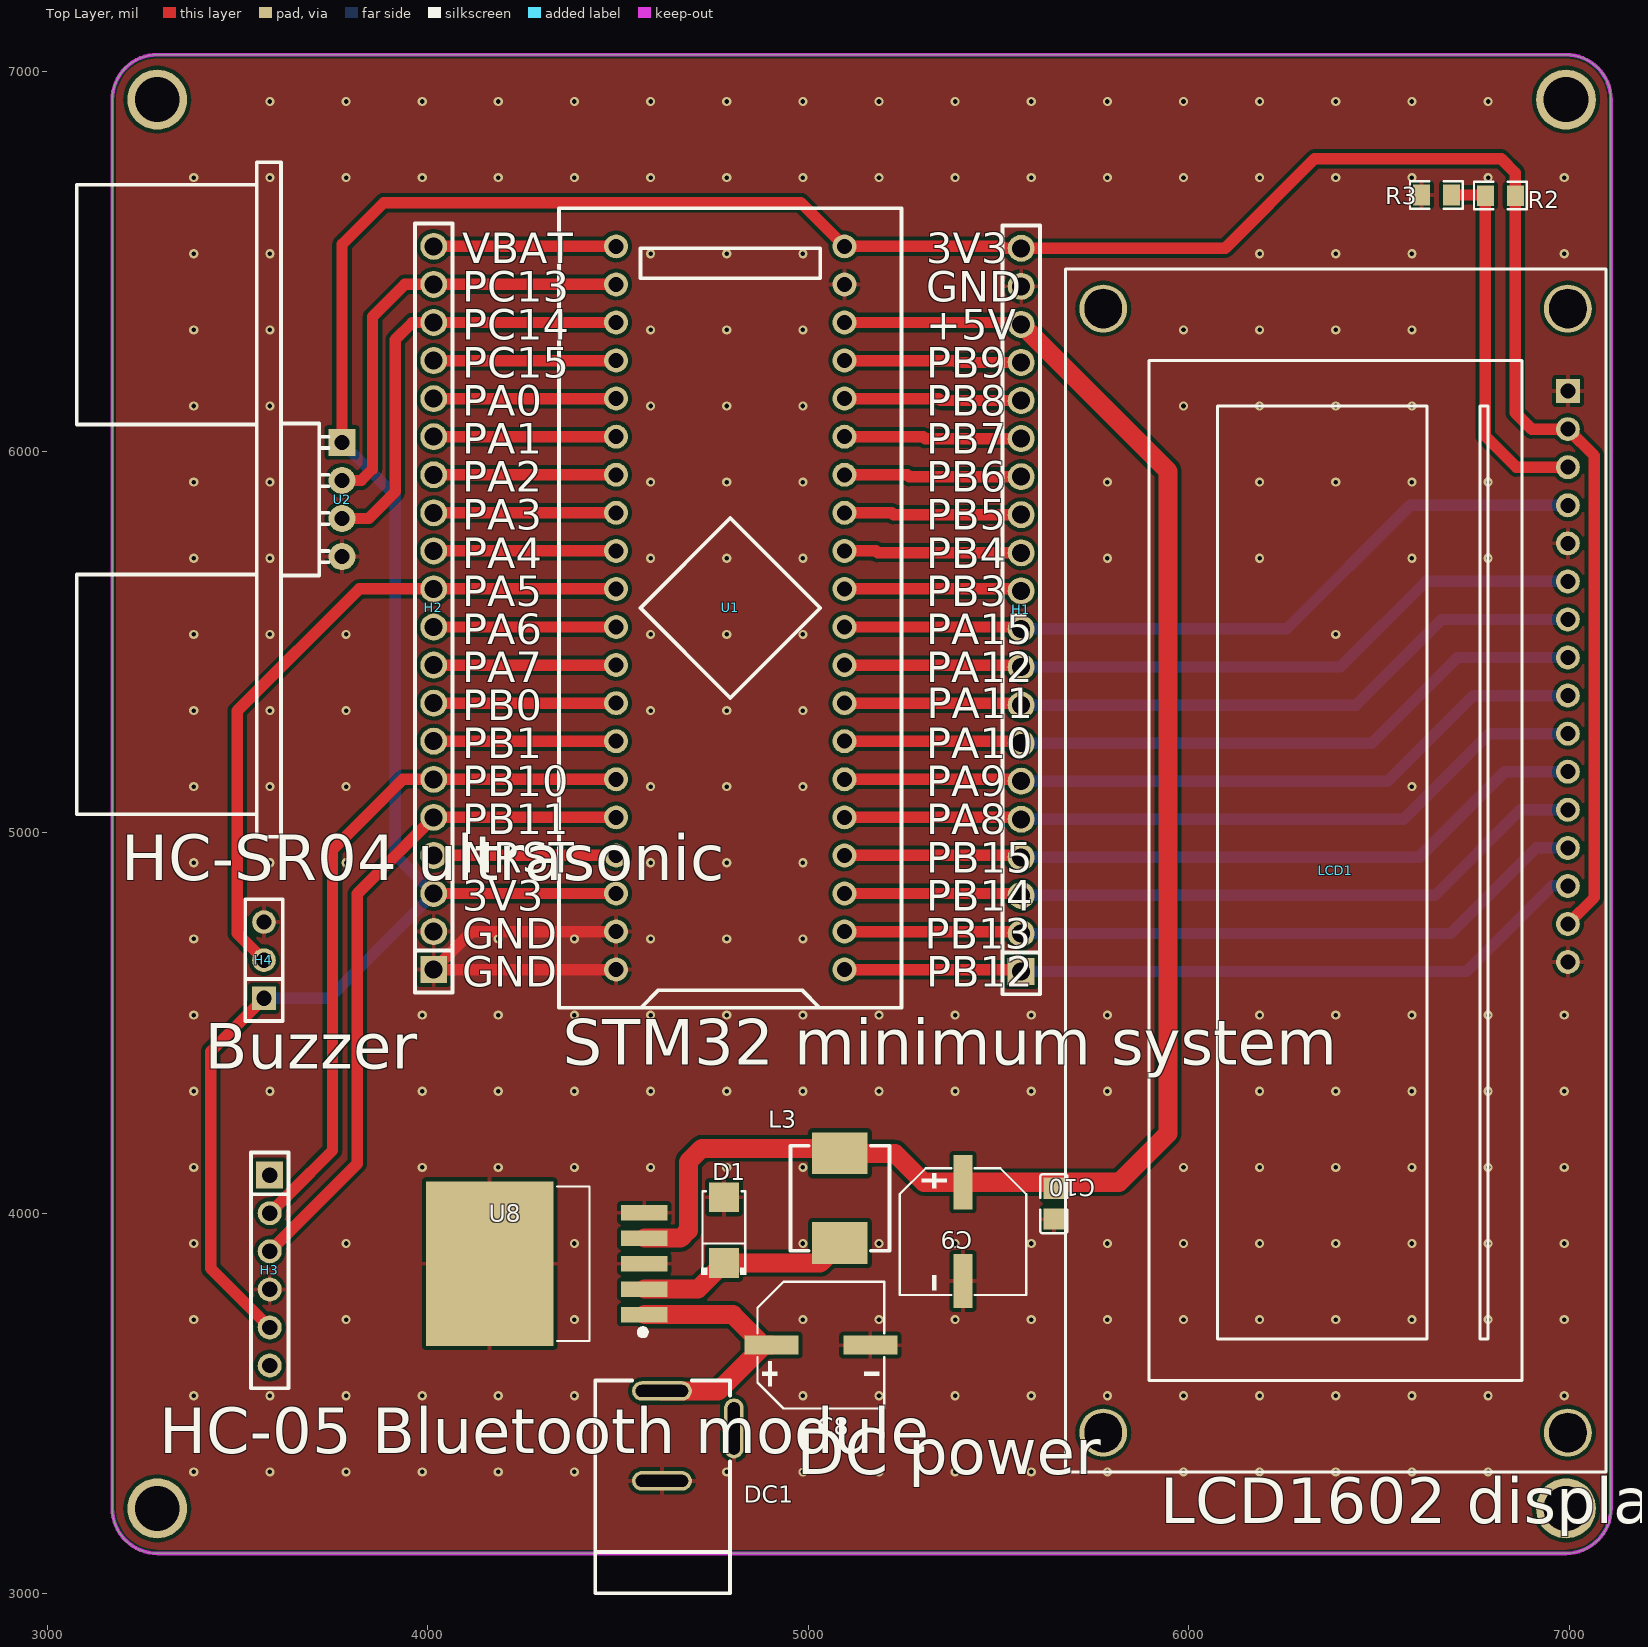
[diagram p0: Top Layer view]
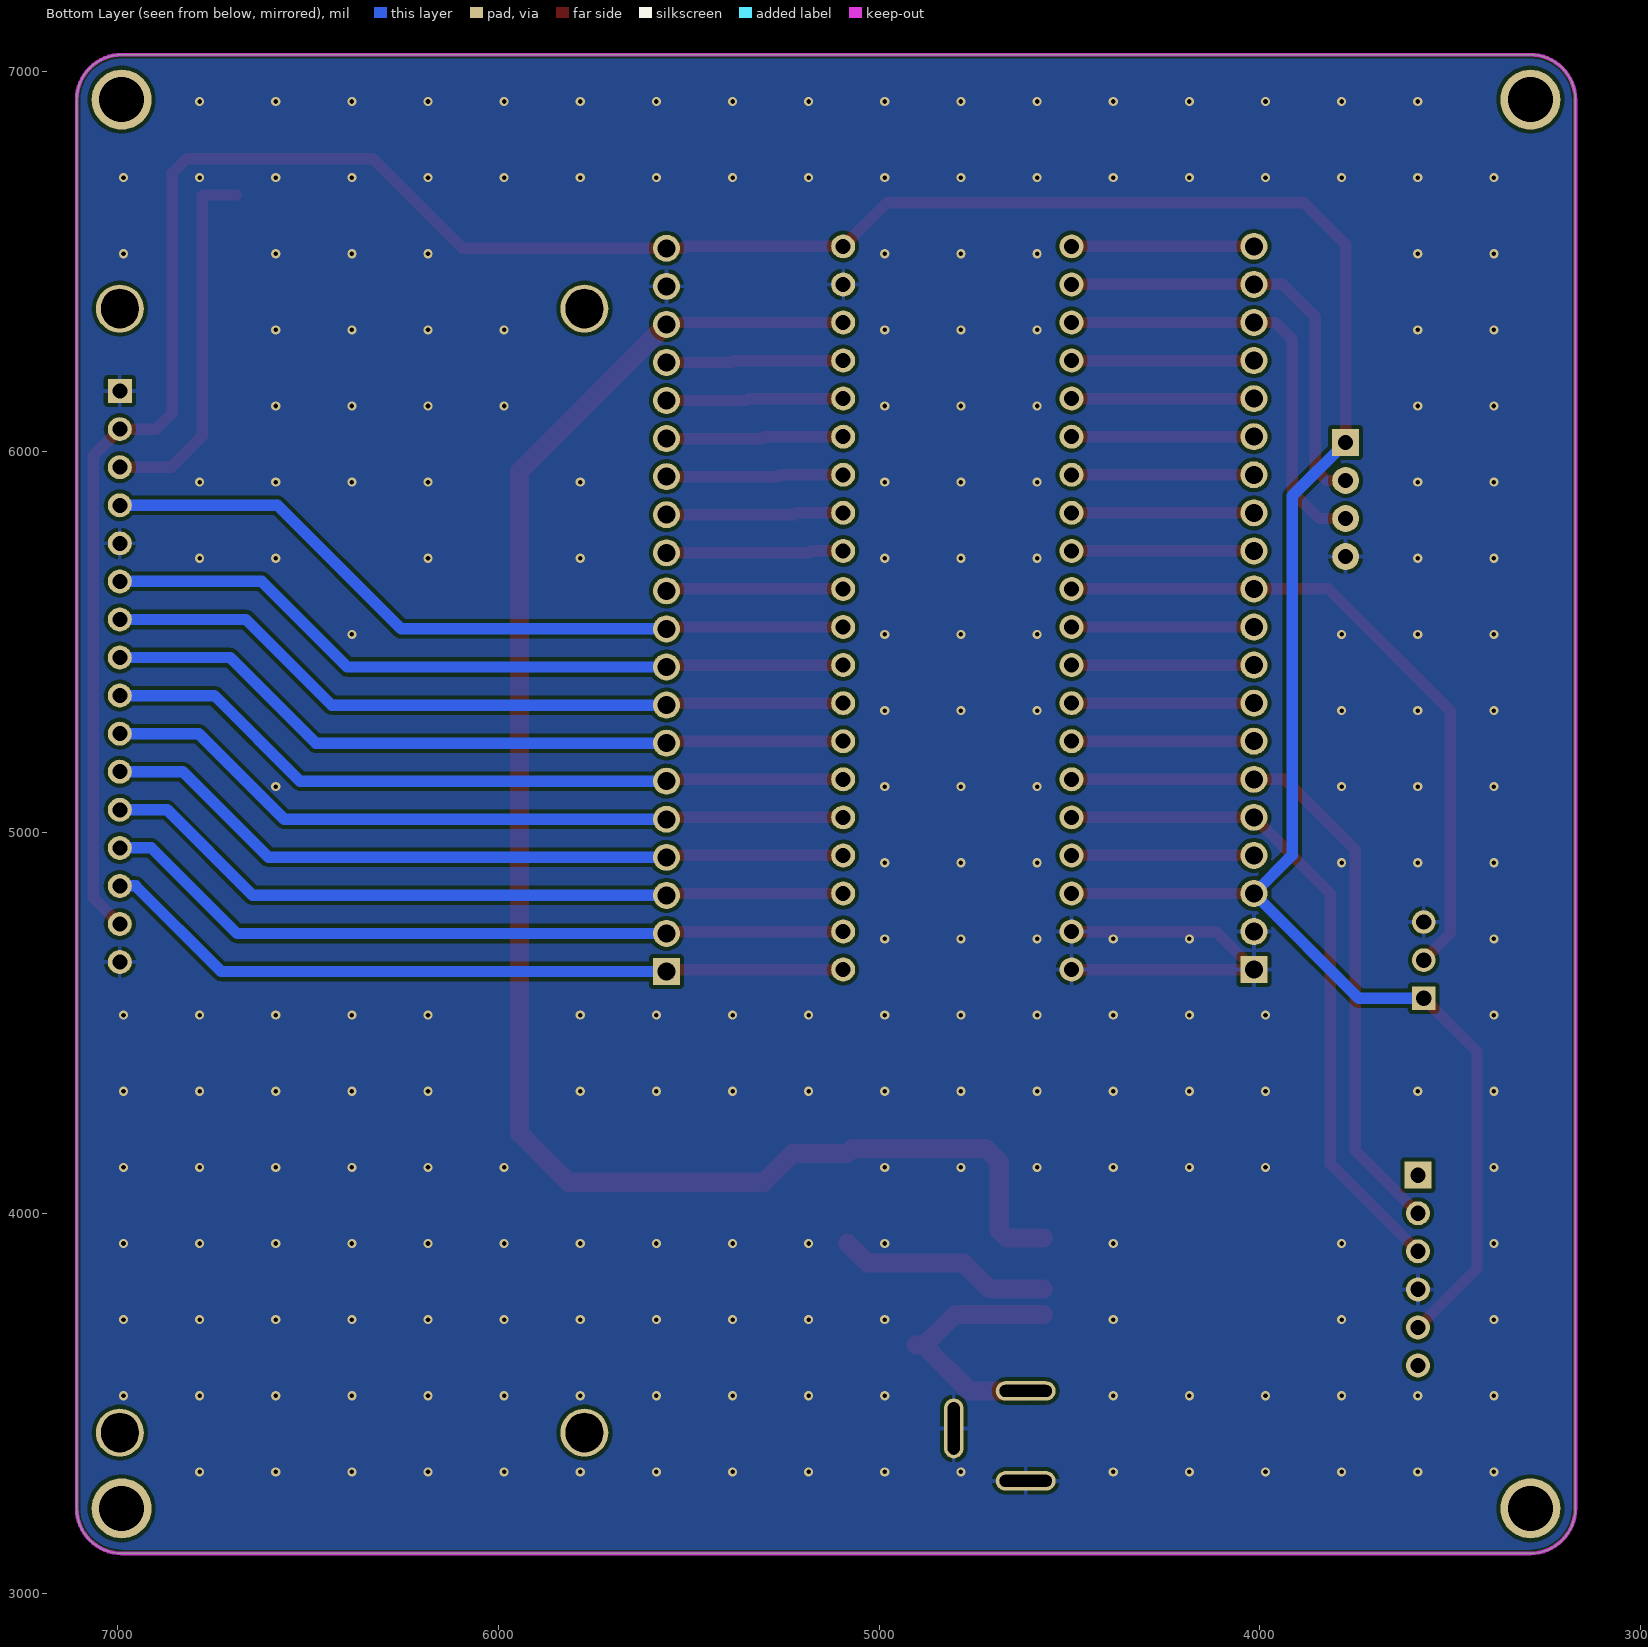
[diagram p1: Bottom Layer view, seen from below]
# Altium PCB MISC89129.pcbdoc
Units mil, origin at the board's own origin, x right, y up, seen from the top; angles counter-clockwise.
Board outline 3937.01 x 3937.01 mil, 2 copper layers (Top Layer, Bottom Layer), stack 62.206 mil thick; 16 components, 40 nets, 140 pads, 222 vias.

## Layer stack, top to bottom
Top Solder Mask Layer: solder mask 0.394, Dk 3.3
Top Layer: signal copper 1.379
Dielectric1: surface 59.449, FR4, Dk 4.5
Bottom Layer: signal copper 1.378
Bottom Solder Mask Layer: solder mask 0.394, Dk 3.3

## Board outline
3289.61,7043.5 ccw(c3289.61,6925.39) 3171.5,6925.39 3171.5,3224.61 ccw(c3289.61,3224.61) 3289.61,3106.5 6990.39,3106.5 ccw(c6990.39,3224.61) 7108.5,3224.61 7108.5,6925.39 ccw(c6990.39,6925.39) 6990.39,7043.5 3289.61,7043.5

## Design rules (kind name [scope] priority, off if disabled: settings)
BoardOutlineClearance copperThickness2oz_1 [All] p2 off: genericclearance=7.99 ignorepadtopadclearanceinfootprint=FALSE except(0: Arc-SplitContinuation Track-SplitContinuation SMDPad-SplitContinuation THPad-SplitContinuation Via-SplitContinuation Fill-SplitContinuation Region-SplitContinuation Poly-SplitContinuation Text-SplitContinuation Hole-SplitContinuation; 5.98: Arc-CutoutEdge Track-CutoutEdge SMDPad-CutoutEdge THPad-CutoutEdge Via-CutoutEdge Text-CutoutEdge; 6.9: Hole-OutlineEdge Hole-CutoutEdge; 10: Poly-OutlineEdge Poly-CutoutEdge; 11.81: Arc-OutlineEdge Track-OutlineEdge SMDPad-OutlineEdge THPad-OutlineEdge Via-OutlineEdge Fill-OutlineEdge Region-OutlineEdge Text-OutlineEdge Fill-CutoutEdge Region-CutoutEdge)
BoardOutlineClearance Plane_innerPlane_1 [All] p4 off: genericclearance=4.02 ignorepadtopadclearanceinfootprint=FALSE except(0: Arc-SplitContinuation Track-SplitContinuation SMDPad-SplitContinuation THPad-SplitContinuation Via-SplitContinuation Fill-SplitContinuation Region-SplitContinuation Poly-SplitContinuation Text-SplitContinuation Hole-SplitContinuation; 5.98: Arc-CutoutEdge Track-CutoutEdge SMDPad-CutoutEdge THPad-CutoutEdge Via-CutoutEdge Text-CutoutEdge; 6.9: Hole-OutlineEdge Hole-CutoutEdge; 10: Poly-OutlineEdge Poly-CutoutEdge; 11.81: Arc-OutlineEdge Track-OutlineEdge SMDPad-OutlineEdge THPad-OutlineEdge Via-OutlineEdge Fill-OutlineEdge Region-OutlineEdge Text-OutlineEdge Fill-CutoutEdge Region-CutoutEdge)
BoardOutlineClearance Copper_copperRegion_1 [All] p6 off: genericclearance=4.02 ignorepadtopadclearanceinfootprint=FALSE except(0: Arc-SplitContinuation Track-SplitContinuation SMDPad-SplitContinuation THPad-SplitContinuation Via-SplitContinuation Fill-SplitContinuation Region-SplitContinuation Poly-SplitContinuation Text-SplitContinuation Hole-SplitContinuation; 5.98: Arc-CutoutEdge Track-CutoutEdge SMDPad-CutoutEdge THPad-CutoutEdge Via-CutoutEdge Text-CutoutEdge; 6.9: Hole-OutlineEdge Hole-CutoutEdge; 10: Poly-OutlineEdge Poly-CutoutEdge; 11.81: Arc-OutlineEdge Track-OutlineEdge SMDPad-OutlineEdge THPad-OutlineEdge Via-OutlineEdge Fill-OutlineEdge Region-OutlineEdge Text-OutlineEdge Fill-CutoutEdge Region-CutoutEdge)
BoardOutlineClearance copperThickness1oz_1 [All] p8: genericclearance=4.02 ignorepadtopadclearanceinfootprint=FALSE except(0: Arc-SplitContinuation Track-SplitContinuation SMDPad-SplitContinuation THPad-SplitContinuation Via-SplitContinuation Fill-SplitContinuation Region-SplitContinuation Poly-SplitContinuation Text-SplitContinuation Hole-SplitContinuation; 5.98: Arc-CutoutEdge Track-CutoutEdge SMDPad-CutoutEdge THPad-CutoutEdge Via-CutoutEdge Text-CutoutEdge; 6.9: Hole-OutlineEdge Hole-CutoutEdge; 10: Poly-OutlineEdge Poly-CutoutEdge; 11.81: Arc-OutlineEdge Track-OutlineEdge SMDPad-OutlineEdge THPad-OutlineEdge Via-OutlineEdge Fill-OutlineEdge Region-OutlineEdge Text-OutlineEdge Fill-CutoutEdge Region-CutoutEdge)
Clearance copperThickness2oz [All] p1 off: gap=7.99 ignorepadtopadclearanceinfootprint=FALSE except(5.98: SMDPad-Track SMDPad-SMDPad THPad-Track SMDPad-THPad THPad-THPad Track-Via SMDPad-Via THPad-Via Via-Via Fill-SMDPad Region-SMDPad Fill-THPad Region-THPad Fill-Via Region-Via Fill-Fill Fill-Region Region-Region Arc-Track Arc-SMDPad Arc-THPad Arc-Via Fill-Arc Region-Arc Arc-Arc Text-Track SMDPad-Text Text-THPad Text-Via Fill-Text Region-Text Arc-Text Text-Text; 6.9: Hole-Track Hole-SMDPad Hole-THPad Hole-Via Fill-Hole Region-Hole Hole-Arc Hole-Text; 10: Poly-Track Poly-SMDPad Poly-THPad Poly-Via Poly-Fill Poly-Region Poly-Poly Poly-Arc Poly-Text Poly-Hole; 11.81: Fill-Track Region-Track)
Clearance Plane_innerPlane [All] p3 off: gap=4.02 ignorepadtopadclearanceinfootprint=FALSE except(5.98: SMDPad-Track SMDPad-SMDPad THPad-Track SMDPad-THPad THPad-THPad Track-Via SMDPad-Via THPad-Via Via-Via Fill-SMDPad Region-SMDPad Fill-THPad Region-THPad Fill-Via Region-Via Fill-Fill Fill-Region Region-Region Arc-Track Arc-SMDPad Arc-THPad Arc-Via Fill-Arc Region-Arc Arc-Arc Text-Track SMDPad-Text Text-THPad Text-Via Fill-Text Region-Text Arc-Text Text-Text; 6.9: Hole-Track Hole-SMDPad Hole-THPad Hole-Via Fill-Hole Region-Hole Hole-Arc Hole-Text; 10: Poly-Track Poly-SMDPad Poly-THPad Poly-Via Poly-Fill Poly-Region Poly-Poly Poly-Arc Poly-Text Poly-Hole; 11.81: Fill-Track Region-Track)
Clearance Copper_copperRegion [All] p5 off: gap=4.02 ignorepadtopadclearanceinfootprint=FALSE except(5.98: SMDPad-Track SMDPad-SMDPad THPad-Track SMDPad-THPad THPad-THPad Track-Via SMDPad-Via THPad-Via Via-Via Fill-SMDPad Region-SMDPad Fill-THPad Region-THPad Fill-Via Region-Via Fill-Fill Fill-Region Region-Region Arc-Track Arc-SMDPad Arc-THPad Arc-Via Fill-Arc Region-Arc Arc-Arc Text-Track SMDPad-Text Text-THPad Text-Via Fill-Text Region-Text Arc-Text Text-Text; 6.9: Hole-Track Hole-SMDPad Hole-THPad Hole-Via Fill-Hole Region-Hole Hole-Arc Hole-Text; 10: Poly-Track Poly-SMDPad Poly-THPad Poly-Via Poly-Fill Poly-Region Poly-Poly Poly-Arc Poly-Text Poly-Hole; 11.81: Fill-Track Region-Track)
Clearance copperThickness1oz [All] p7: gap=4.02 ignorepadtopadclearanceinfootprint=FALSE except(5.98: SMDPad-Track SMDPad-SMDPad THPad-Track SMDPad-THPad THPad-THPad Track-Via SMDPad-Via THPad-Via Via-Via Fill-SMDPad Region-SMDPad Fill-THPad Region-THPad Fill-Via Region-Via Fill-Fill Fill-Region Region-Region Arc-Track Arc-SMDPad Arc-THPad Arc-Via Fill-Arc Region-Arc Arc-Arc Text-Track SMDPad-Text Text-THPad Text-Via Fill-Text Region-Text Arc-Text Text-Text; 6.9: Hole-Track Hole-SMDPad Hole-THPad Hole-Via Fill-Hole Region-Hole Hole-Arc Hole-Text; 10: Poly-Track Poly-SMDPad Poly-THPad Poly-Via Poly-Fill Poly-Region Poly-Poly Poly-Arc Poly-Text Poly-Hole; 11.81: Fill-Track Region-Track)
DiffPairsRouting differentialPair [All] p1: maxlimit=6 minlimit=6 mostfreqgap=6 toplayer_minwidth=5 toplayer_prefwidth=10 toplayer_maxwidth=100 toplayer_mingap=6 toplayer_prefgap=6 toplayer_maxgap=6 bottomlayer_minwidth=5 bottomlayer_prefwidth=10 bottomlayer_maxwidth=100 bottomlayer_mingap=6 bottomlayer_prefgap=6 bottomlayer_maxgap=6 maxuncoupledlength=10
HoleToHoleClearance otherClearance [All] p1: gap=11.81 allowstackedmicrovias=TRUE
Length netLength [All] p1: minlimit=0 maxlimit=0
PasteMaskExpansion pasteMaskExpansion [All] p1: expansion=0
PlaneConnect innerPlane [All] p1: planeconnectstyle=Relief reliefexpansion=20 reliefentries=4 reliefconductorwidth=10 reliefairgap=10
PolygonConnect copperRegion [All] p1: connectstyle=Relief reliefconductorwidth=10 reliefentries=4 polygonreliefangle="90 Angle" airgapwidth=10 via.connectstyle=Relief via.reliefconductorwidth=10 via.reliefentries=4 via.polygonreliefangle="90 Angle" via.airgapwidth=10
RoutingVias viaSize [All] p1: holewidth=12.01 width=24.02 viastyle="Through Hole" minholewidth=11.81 minwidth=19.68 maxholewidth=248.03 maxwidth=393.7
SolderMaskExpansion solderMaskExpansion [IsVia] p1: expansion=-1000 istentingtop=TRUE
SolderMaskExpansion solderMaskExpansion [All] p2: expansion=2 istentingtop=FALSE
Width copperThickness2oz_2 [All] p1 off: maxlimit=100 minlimit=8 preferedwidth=10
Width copperThickness1oz_2 [All] p2: maxlimit=100 minlimit=5 preferedwidth=10

## Components (designator, comment, footprint, x,y, rotation, side; value= is the part's Value field where it differs from the comment)
C8 "" CAP-SMD_BD8.0-L8.3-W8.3-RD 5033.1,3653.46 r180 top
C9 "" CAP-SMD_BD8.0-L8.3-W8.3-RD 5406.18,3951.73 r90 top
C10 "" C0805 5645,4025 r270 top
D1 "" SMA_L4.3-W2.6-LS5.2-RD 4778.1,3955.46 r90 top
DC1 "" DC-2.0 4605,3410 r270 top
H1 "" HDR-TH_20P-P2.54-V-F 5559.16,5585 r90 top
H2 "" HDR-TH_20P-P2.54-V-F 4015.95,5590 r90 top
H3 "" HDR-TH_6P-P2.54-V-F 3585,3850 r270 top
H4 "" HDR-TH_3P-P2.54-V-F 3570,4665 r90 top
L3 "" IND-SMD_L7.0-W6.6 5083.1,4039.46 r90 top
LCD1 "LMB162ADC" LCD1602 6385,4900 r270 top
R2 "10K" R0805 6817.76,6673.32 r0 top
R3 "1K" R0805 6650,6675 r0 top
U1 "STM32F103C8T6-Card" CONN-TH_L53.3-W22.9_STM32F103C8T6-CARD 4795,5590 r90 top
U2 "HC-SR04" TH_HC-SR04V 3775,5875 r270 top
U8 "LM2596S-5.0" TO-263-5_L10.2-W8.9-P1.70-BR 4365.96,3867.46 r0 top

## Footprints (in the part's own frame and the unit in brackets; to place one, negate y for a bottom-side part, rotate by r counter-clockwise, add the part's x,y. Pads: shape width x height; smd on the part's side, far side on the other; paste and mask are expansions set on the pad)
C0805 [mm]
  rect 1.41x1.35 smd paste-100 mask+0.051: 1(-1.03,0) 2(1.03,0)
  silkscreen extent -1.96,-0.9 1.96,0.9
CAP-SMD_BD8.0-L8.3-W8.3-RD [mm]
  rect 3.61x1.26 smd paste+0 mask+0.051: 1(3.295,0) 2(-3.295,0)
  silkscreen extent -4.23,-4.23 4.23,4.23
CONN-TH_L53.3-W22.9_STM32F103C8T6-CARD [mm]
  round 1.6 hole 1: 1(-24.13,-7.62) 2(-21.59,-7.62) 3(-19.05,-7.62) 4(-16.51,-7.62) 5(-13.97,-7.62) 6(-11.43,-7.62) 7(-8.89,-7.62) 8(-6.35,-7.62) 9(-3.81,-7.62) 10(-1.27,-7.62) 11(1.27,-7.62) 12(3.81,-7.62) 13(6.35,-7.62) 14(8.89,-7.62) 15(11.43,-7.62) 16(13.97,-7.62) 17(16.51,-7.62) 18(19.05,-7.62) 19(21.59,-7.62) 20(24.13,-7.62) 21(24.13,7.62) 22(21.59,7.62) 23(19.05,7.62) 24(16.51,7.62) 25(13.97,7.62) 26(11.43,7.62) 27(8.89,7.62) 28(6.35,7.62) 29(3.81,7.62) 30(1.27,7.62) 31(-1.27,7.62) 32(-3.81,7.62) 33(-6.35,7.62) 34(-8.89,7.62) 35(-11.43,7.62) 36(-13.97,7.62) 37(-16.51,7.62) 38(-19.05,7.62) 39(-21.59,7.62) 40(-24.13,7.62)
  silkscreen extent -26.67,-11.43 26.67,11.43
DC-2.0 [mil]
  oval 157.5x51.2 hole 31.5 slot 137.8 at 0 deg paste+0 mask+2: 2(-24.7,199.5)
  oval 51.2x157.5 hole 31.5 slot 137.8 at 90 deg paste+0 mask+2: 3(113.1,10.5) 4(-123.1,10.5)
  silkscreen extent -151,-165 408,190
HDR-TH_3P-P2.54-V-F [mil]
  rect 62x62 hole 40.16: 1(-100,0)
  round 62 hole 40.16: 2(0,0) 3(100,0)
  silkscreen extent -160,-49 160,49
HDR-TH_6P-P2.54-V-F [mm]
  rect 1.8x1.8 hole 1.02: 1(-6.35,0)
  round 1.6 hole 1.02: 2(-3.81,0) 3(-1.27,0) 4(1.27,0) 5(3.81,0) 6(6.35,0)
  silkscreen extent -7.87,-1.25 7.87,1.25
HDR-TH_20P-P2.54-V-F [mm]
  rect 1.8x1.8 hole 1.2: 1(-24.13,0)
  round 1.8 hole 1.2: 2(-21.59,0) 3(-19.05,0) 4(-16.51,0) 5(-13.97,0) 6(-11.43,0) 7(-8.89,0) 8(-6.35,0) 9(-3.81,0) 10(-1.27,0) 11(1.27,0) 12(3.81,0) 13(6.35,0) 14(8.89,0) 15(11.43,0) 16(13.97,0) 17(16.51,0) 18(19.05,0) 19(21.59,0) 20(24.13,0)
  silkscreen extent -25.65,-1.25 25.65,1.25
IND-SMD_L7.0-W6.6 [mil]
  rect 110.2x145.7 smd paste+0 mask+2: 1(-118.1,0) 2(118.1,0)
  silkscreen extent -138,-130 138,130
LCD1602 [mm]
  round 3.2 hole 2.5 slot 2.625 at 0 deg: 0(-37.5,-15.5) 0(-37.5,15.5) 0(37.5,-15.5) 0(37.5,15.5)
  rect 1.6x1.6 hole 1: 1(-32,15.5)
  round 1.6 hole 1: 2(-29.46,15.5) 3(-26.92,15.5) 4(-24.38,15.5) 5(-21.84,15.5) 6(-19.3,15.5) 7(-16.76,15.5) 8(-14.22,15.5) 9(-11.68,15.5) 10(-9.14,15.5) 11(-6.6,15.5) 12(-4.06,15.5) 13(-1.52,15.5) 14(1.02,15.5) 15(3.56,15.5) 16(6.1,15.5)
  silkscreen extent -40.13,-18.03 40.13,18.03
R0805 [mm]
  rect 1.133x1.377 smd paste-100 mask+0.051: 1(-1,0) 2(1,0)
  silkscreen extent -1.76,-0.92 1.76,0.92
SMA_L4.3-W2.6-LS5.2-RD [mm]
  rect 2x2 smd paste+0 mask+0.051: 1(-2.2,0) 2(2.2,0)
  silkscreen extent -2.98,-1.5 2.6,1.5
TH_HC-SR04V [mm]
  rect 1.8x1.8 hole 1.001: 1(-3.81,0)
  round 1.8 hole 1.001: 2(-1.27,0) 3(1.27,0) 4(3.81,0)
  silkscreen extent -22.5,-17.7 22.5,-0.89
TO-263-5_L10.2-W8.9-P1.70-BR [mm]
  rect 3.083x1.02 smd: 1(5.16,-3.4) 2(5.16,-1.7) 3(5.16,0) 4(5.16,1.7) 5(5.16,3.4)
  rect 8.5x11 smd: 6(-5.16,0)
  silkscreen extent -0.66,-5.16 5.26,5.16

## Free pads (board coordinates)
  round 157.48 hole 118.11: 1(3289.61,6925.39) 1(3289.61,3224.61) 1(6990.39,6925.39) 1(6990.39,3224.61)

## Via types
v1: diameter 24.02, hole 12, Top Layer to Bottom Layer, 222 vias

## Nets (pads, with @x,y where several pads share a name; then routed paths per layer and width w, separated by ;. In a path a pad name is that pad's centre, name@x,y a point inside that pad or via, vN(x,y) a via of type N, cw(c..) or ccw(c..) an arc to the next point about the centre after c; other vN are vias at no path point)
$1N17012: LCD1.3 R2.1 R3.2 | length 972.1
  Top Layer w30: R3.2 6776.72,6675 R2.1 6778.39,6041.61 6860.16,5959.84 LCD1.3
$1N17040: C8.1 DC1.4 U8.1 | length 685.3
  Top Layer w50: U8.1 4801.4,3733.6 4881.54,3653.46 C8.1@4883.46,3653.46 ; DC1.4 4763.1,3533.1 C8.1@4883.46,3653.46 ; C8.1 C8.1@4883.46,3653.46
$1N17045: D1.1 L3.1 U8.2 | length 564
  Top Layer w50: U8.2 4709.78,3800.53 D1.1 5030.59,3868.85 L3.1
+5V: C9.1 C10.1 H1.18 L3.2 U1.18 U8.4 | length 4413.1
  Top Layer w30: U1.18 H1.18@5554.16,6340
  Top Layer w50: U8.4 4664.39,3934.39 4685,3955 4685,4135 4720.36,4170.36 5070.3,4170.36 L3.2 5227.44,4157.56 5303.55,4081.45 C9.1 5816.45,4081.45 5945,4210 5945,5949.16 H1.18
GND: C8.2 C9.2 C10.2 D1.2 DC1.2 DC1.3 H1.19 H2.1 H2.2 H3.4 H4.3 LCD1.1 LCD1.5 LCD1.16 R3.1 U1.19 U1.39 U1.40 U2.4 U8.3 U8.5 U8.6 | length 999.5
  Top Layer w30: U1.40 H2.1 4115.95,4740 U1.39
  other v1: 3385.6,3320.6 3585.6,3320.6 3785.6,3320.6 3985.6,3320.6 4185.6,3320.6 4385.6,3320.6 4785.6,3320.6 4985.6,3320.6 5185.6,3320.6 5385.6,3320.6 5585.6,3320.6 5785.6,3320.6 5985.6,3320.6 6185.6,3320.6 6385.6,3320.6 6585.6,3320.6 6785.6,3320.6 3385.6,3520.6 3585.6,3520.6 3785.6,3520.6 3985.6,3520.6 4185.6,3520.6 4385.6,3520.6 4985.6,3520.6 5185.6,3520.6 5385.6,3520.6 5585.6,3520.6 5785.6,3520.6 5985.6,3520.6 6185.6,3520.6 6385.6,3520.6 6585.6,3520.6 6785.6,3520.6 6985.6,3520.6 3385.6,3720.6 3785.6,3720.6 4385.6,3720.6 4985.6,3720.6 5185.6,3720.6 5385.6,3720.6 5585.6,3720.6 5785.6,3720.6 5985.6,3720.6 6185.6,3720.6 6385.6,3720.6 6585.6,3720.6 6785.6,3720.6 6985.6,3720.6 3385.6,3920.6 3785.6,3920.6 4385.6,3920.6 4985.6,3920.6 5185.6,3920.6 5385.6,3920.6 5585.6,3920.6 5785.6,3920.6 5985.6,3920.6 6185.6,3920.6 6385.6,3920.6 6585.6,3920.6 6785.6,3920.6 6985.6,3920.6 3385.6,4120.6 3985.6,4120.6 4185.6,4120.6 4385.6,4120.6 4585.6,4120.6 4785.6,4120.6 4985.6,4120.6 5985.6,4120.6 6185.6,4120.6 6385.6,4120.6 6585.6,4120.6 6785.6,4120.6 6985.6,4120.6 3385.6,4320.6 3585.6,4320.6 3985.6,4320.6 4185.6,4320.6 4385.6,4320.6 4585.6,4320.6 4785.6,4320.6 4985.6,4320.6 5185.6,4320.6 5385.6,4320.6 5585.6,4320.6 5785.6,4320.6 6185.6,4320.6 6385.6,4320.6 6585.6,4320.6 6785.6,4320.6 6985.6,4320.6 3385.6,4520.6 3985.6,4520.6 4185.6,4520.6 4385.6,4520.6 4585.6,4520.6 4785.6,4520.6 4985.6,4520.6 5185.6,4520.6 5385.6,4520.6 5585.6,4520.6 5785.6,4520.6 6185.6,4520.6 6385.6,4520.6 6585.6,4520.6 6785.6,4520.6 6985.6,4520.6 3385.6,4720.6 4185.6,4720.6 4385.6,4720.6 4585.6,4720.6 4785.6,4720.6 4985.6,4720.6 3385.6,4920.6 3585.6,4920.6 3785.6,4920.6 4585.6,4920.6 4785.6,4920.6 4985.6,4920.6 3385.6,5120.6 3585.6,5120.6 3785.6,5120.6 4585.6,5120.6 4785.6,5120.6 4985.6,5120.6 6585.6,5120.6 3385.6,5320.6 3585.6,5320.6 3785.6,5320.6 4585.6,5320.6 4785.6,5320.6 4985.6,5320.6 3385.6,5520.6 3585.6,5520.6 3785.6,5520.6 4585.6,5520.6 4785.6,5520.6 4985.6,5520.6 6385.6,5520.6 3385.6,5720.6 3585.6,5720.6 4585.6,5720.6 4785.6,5720.6 4985.6,5720.6 5785.6,5720.6 6185.6,5720.6 6585.6,5720.6 6785.6,5720.6 3385.6,5920.6 3585.6,5920.6 4585.6,5920.6 4785.6,5920.6 4985.6,5920.6 5785.6,5920.6 6185.6,5920.6 6385.6,5920.6 6585.6,5920.6 6785.6,5920.6 3385.6,6120.6 3585.6,6120.6 4585.6,6120.6 4785.6,6120.6 4985.6,6120.6 5985.6,6120.6 6185.6,6120.6 6385.6,6120.6 6585.6,6120.6 3385.6,6320.6 3585.6,6320.6 4585.6,6320.6 4785.6,6320.6 4985.6,6320.6 5985.6,6320.6 6185.6,6320.6 6385.6,6320.6 6585.6,6320.6 3385.6,6520.6 3585.6,6520.6 4585.6,6520.6 4785.6,6520.6 4985.6,6520.6 6185.6,6520.6 6385.6,6520.6 6585.6,6520.6 6985.6,6520.6 3385.6,6720.6 3585.6,6720.6 3785.6,6720.6 3985.6,6720.6 4185.6,6720.6 4385.6,6720.6 4585.6,6720.6 4785.6,6720.6 4985.6,6720.6 5185.6,6720.6 5385.6,6720.6 5585.6,6720.6 5785.6,6720.6 5985.6,6720.6 6185.6,6720.6 6385.6,6720.6 6585.6,6720.6 6785.6,6720.6 6985.6,6720.6 3585.6,6920.6 3785.6,6920.6 3985.6,6920.6 4185.6,6920.6 4385.6,6920.6 4585.6,6920.6 4785.6,6920.6 4985.6,6920.6 5185.6,6920.6 5385.6,6920.6 5585.6,6920.6 5785.6,6920.6 5985.6,6920.6 6185.6,6920.6 6385.6,6920.6 6585.6,6920.6 6785.6,6920.6
NRST: H2.4 U1.37 | length 479
  Top Layer w30: H2.4 U1.37
PA0: H2.16 U1.25 | length 479
  Top Layer w30: H2.16 U1.25
PA1: H2.15 U1.26 | length 479
  Top Layer w30: H2.15 U1.26
PA2: H2.14 U1.27 | length 479
  Top Layer w30: H2.14 U1.27
PA3: H2.13 U1.28 | length 479
  Top Layer w30: H2.13 U1.28
PA4: H2.12 U1.29 | length 479
  Top Layer w30: H2.12 U1.29
PA5: H2.11 H4.2 U1.30 | length 1811.5
  Top Layer w30: H4.2 3500,4735 3500,5320 3820,5640 H2.11 U1.30
PA6: H2.10 U1.31 | length 479
  Top Layer w30: H2.10 U1.31
PA7: H2.9 U1.32 | length 479
  Top Layer w30: H2.9 U1.32
PA8: H1.5 LCD1.10 U1.5 | length 1995.4
  Top Layer w30: U1.5 5554.16,5040 H1.5
  Bottom Layer w30: H1.5 6563.22,5035 6788.06,5259.84 LCD1.10
PA9: H1.6 LCD1.9 U1.6 | length 1995.4
  Top Layer w30: U1.6 5554.16,5140 H1.6
  Bottom Layer w30: H1.6 6521.8,5135 6746.64,5359.84 LCD1.9
PA10: H1.7 LCD1.8 U1.7 | length 1995.4
  Top Layer w30: U1.7 5554.16,5240 H1.7
  Bottom Layer w30: H1.7 6480.38,5235 6705.22,5459.84 LCD1.8
PA11: H1.8 LCD1.7 U1.8 | length 1995.4
  Top Layer w30: U1.8 5554.16,5340 H1.8
  Bottom Layer w30: H1.8 6438.95,5335 6663.79,5559.84 LCD1.7
PA12: H1.9 LCD1.6 U1.9 | length 1995.4
  Top Layer w30: U1.9 5554.16,5440 H1.9
  Bottom Layer w30: H1.9 6397.53,5435 6622.37,5659.84 LCD1.6
PA15: H1.10 LCD1.4 U1.10 | length 2036.9
  Top Layer w30: U1.10 5554.16,5540 H1.10
  Bottom Layer w30: H1.10 6256.11,5535 6580.95,5859.84 LCD1.4
PB0: H2.8 U1.33 | length 479
  Top Layer w30: H2.8 U1.33
PB1: H2.7 U1.34 | length 479
  Top Layer w30: H2.7 U1.34
PB3: H1.11 U1.11 | length 466.2
  Top Layer w30: U1.11 5554.16,5640 H1.11
PB4: H1.12 U1.12 | length 466.2
  Top Layer w30: U1.12 5177.35,5740 5182.36,5735 H1.12
PB5: H1.13 U1.13 | length 466.2
  Top Layer w30: U1.13 5218.78,5840 5223.78,5835 H1.13
PB6: H1.14 U1.14 | length 466.2
  Top Layer w30: U1.14 5260.2,5940 5265.2,5935 H1.14
PB7: H1.15 U1.15 | length 466.2
  Top Layer w30: U1.15 5301.62,6040 5306.62,6035 H1.15
PB8: H1.16 U1.16 | length 466.2
  Top Layer w30: U1.16 5343.04,6140 5348.04,6135 H1.16
PB9: H1.17 U1.17 | length 466.2
  Top Layer w30: U1.17 5384.46,6240 5389.46,6235 H1.17
PB10: H2.6 H3.2 U1.35 | length 1845
  Top Layer w30: H3.2 3632.18,4047.18 ccw(c3620.43,4064.57) 3637.82,4052.82 3750,4165 3750,4955 3935,5140 H2.6 U1.35
PB11: H2.5 H3.3 U1.36 | length 1797.6
  Top Layer w30: H3.3 3815,4130 3815,4839.05 H2.5 U1.36
PB12: H1.1 LCD1.14 U1.1 | length 1995.4
  Top Layer w30: U1.1 5554.16,4640 H1.1
  Bottom Layer w30: H1.1 6728.9,4635 6953.74,4859.84 LCD1.14
PB13: H1.2 LCD1.13 U1.2 | length 1995.4
  Top Layer w30: U1.2 5554.16,4740 H1.2
  Bottom Layer w30: H1.2 6687.48,4735 6912.32,4959.84 LCD1.13
PB14: H1.3 LCD1.12 U1.3 | length 1995.4
  Top Layer w30: U1.3 5554.16,4840 H1.3
  Bottom Layer w30: H1.3 6646.06,4835 6870.9,5059.84 LCD1.12
PB15: H1.4 LCD1.11 U1.4 | length 1995.4
  Top Layer w30: U1.4 5554.16,4940 H1.4
  Bottom Layer w30: H1.4 6604.64,4935 6829.48,5159.84 LCD1.11
PC13: H2.19 U1.22 U2.2 | length 1167.6
  Top Layer w30: U2.2 3825,5925 3855,5955 3855,6355 3940,6440 H2.19 U1.22
PC14: H2.18 U1.23 U2.3 | length 1167.6
  Top Layer w30: U2.3 3845,5825 3915,5895 3915,6295 3960,6340 H2.18 U1.23
PC15: H2.17 U1.24 | length 479
  Top Layer w30: H2.17 U1.24
VBAT: H2.20 U1.21 | length 479
  Top Layer w30: H2.20 U1.21
VCC: H1.20 H2.3 H3.5 H4.1 LCD1.2 LCD1.15 R2.2 U1.20 U1.38 U2.1 | length 9264.7
  Top Layer w30: H4.1 3430,4425 3430,3855 H3.5 ; U2.1 3775,6545 3885,6655 4980,6655 U1.20 5508.73,6540 5513.73,6535 H1.20 6095,6535 6330,6770 6820,6770 6857.13,6732.87 R2.2 6857.13,6102.87 6900.16,6059.84 LCD1.2 7065,5990.08 7065,4829.6 LCD1.15 ; H2.3 U1.38
  Bottom Layer w30: H4.1 3740.95,4565 H2.3 3915,4940.95 3915,5885 U2.1
pads on no net: H3.1 H3.6 LCD1.0

## Polygon pours and split planes (outlines as drawn)
GND on Bottom Layer (solid, remove dead copper, pour order 2): 3100,7165 3100,3000 7275,3000 7275,7165
GND on Top Layer (solid, remove dead copper, pour order 0): 3000,7145 3000,3075 7385,3075 7385,7145

## Keep-outs
Board Outline Layer:
  the board outline again, w10

## Silkscreen, mask and mechanical layers (free items; w line width, h text height)
Top Silkscreen Layer:
  text "VBAT" at 4090.95,6495 h80
  text "3V3" at 5309.16,6495 h80
  text "PC13" at 4090.95,6395 h80
  text "GND" at 5309.16,6395 h80
  text "PC14" at 4090.95,6295 h80
  text "+5V" at 5309.16,6295 h80
  text "PC15" at 4090.95,6195 h80
  text "PB9" at 5309.16,6195 h80
  text "PA0" at 4090.95,6095 h80
  text "PB8" at 5309.16,6095 h80
  text "PA1" at 4090.95,5995 h80
  text "PB7" at 5309.16,5995 h80
  text "PA2" at 4090.95,5895 h80
  text "PB6" at 5309.16,5895 h80
  text "PA3" at 4090.95,5795 h80
  text "PB5" at 5309.16,5795 h80
  text "PA4" at 4090.95,5695 h80
  text "PB4" at 5309.16,5695 h80
  text "PA5" at 4090.95,5595 h80
  text "PB3" at 5309.16,5595 h80
  text "PA6" at 4090.95,5495 h80
  text "PA15" at 5309.16,5495 h80
  text "PA7" at 4090.95,5395 h80
  text "PA12" at 5309.16,5395 h80
  text "PA11" at 5310.95,5300 h80
  text "PB0" at 4090.95,5295 h80
  text "PB1" at 4090.95,5195 h80
  text "PA10" at 5309.16,5195 h80
  text "PB10" at 4090.95,5095 h80
  text "PA9" at 5309.16,5095 h80
  text "PB11" at 4090.95,4995 h80
  text "PA8" at 5309.16,4995 h80
  text "NRST" at 4090.95,4895 h80
  text "PB15" at 5309.16,4895 h80
  text "HC-SR04 ultrasonic" at 3195,4875 h120
  text "3V3" at 4090.95,4795 h80
  text "PB14" at 5309.16,4795 h80
  text "GND" at 4090.95,4695 h80
  text "PB13" at 5305.95,4695 h80
  text "GND" at 4090.95,4595 h80
  text "PB12" at 5309.16,4595 h80
  text "STM32 minimum system" at 4355,4390 h120
  text "Buzzer" at 3415,4380 h120
  text "HC-05 Bluetooth module" at 3295,3370 h120
  text "DC power" at 4970,3315 h120
  text "LCD1602 display" at 5925,3185 h120